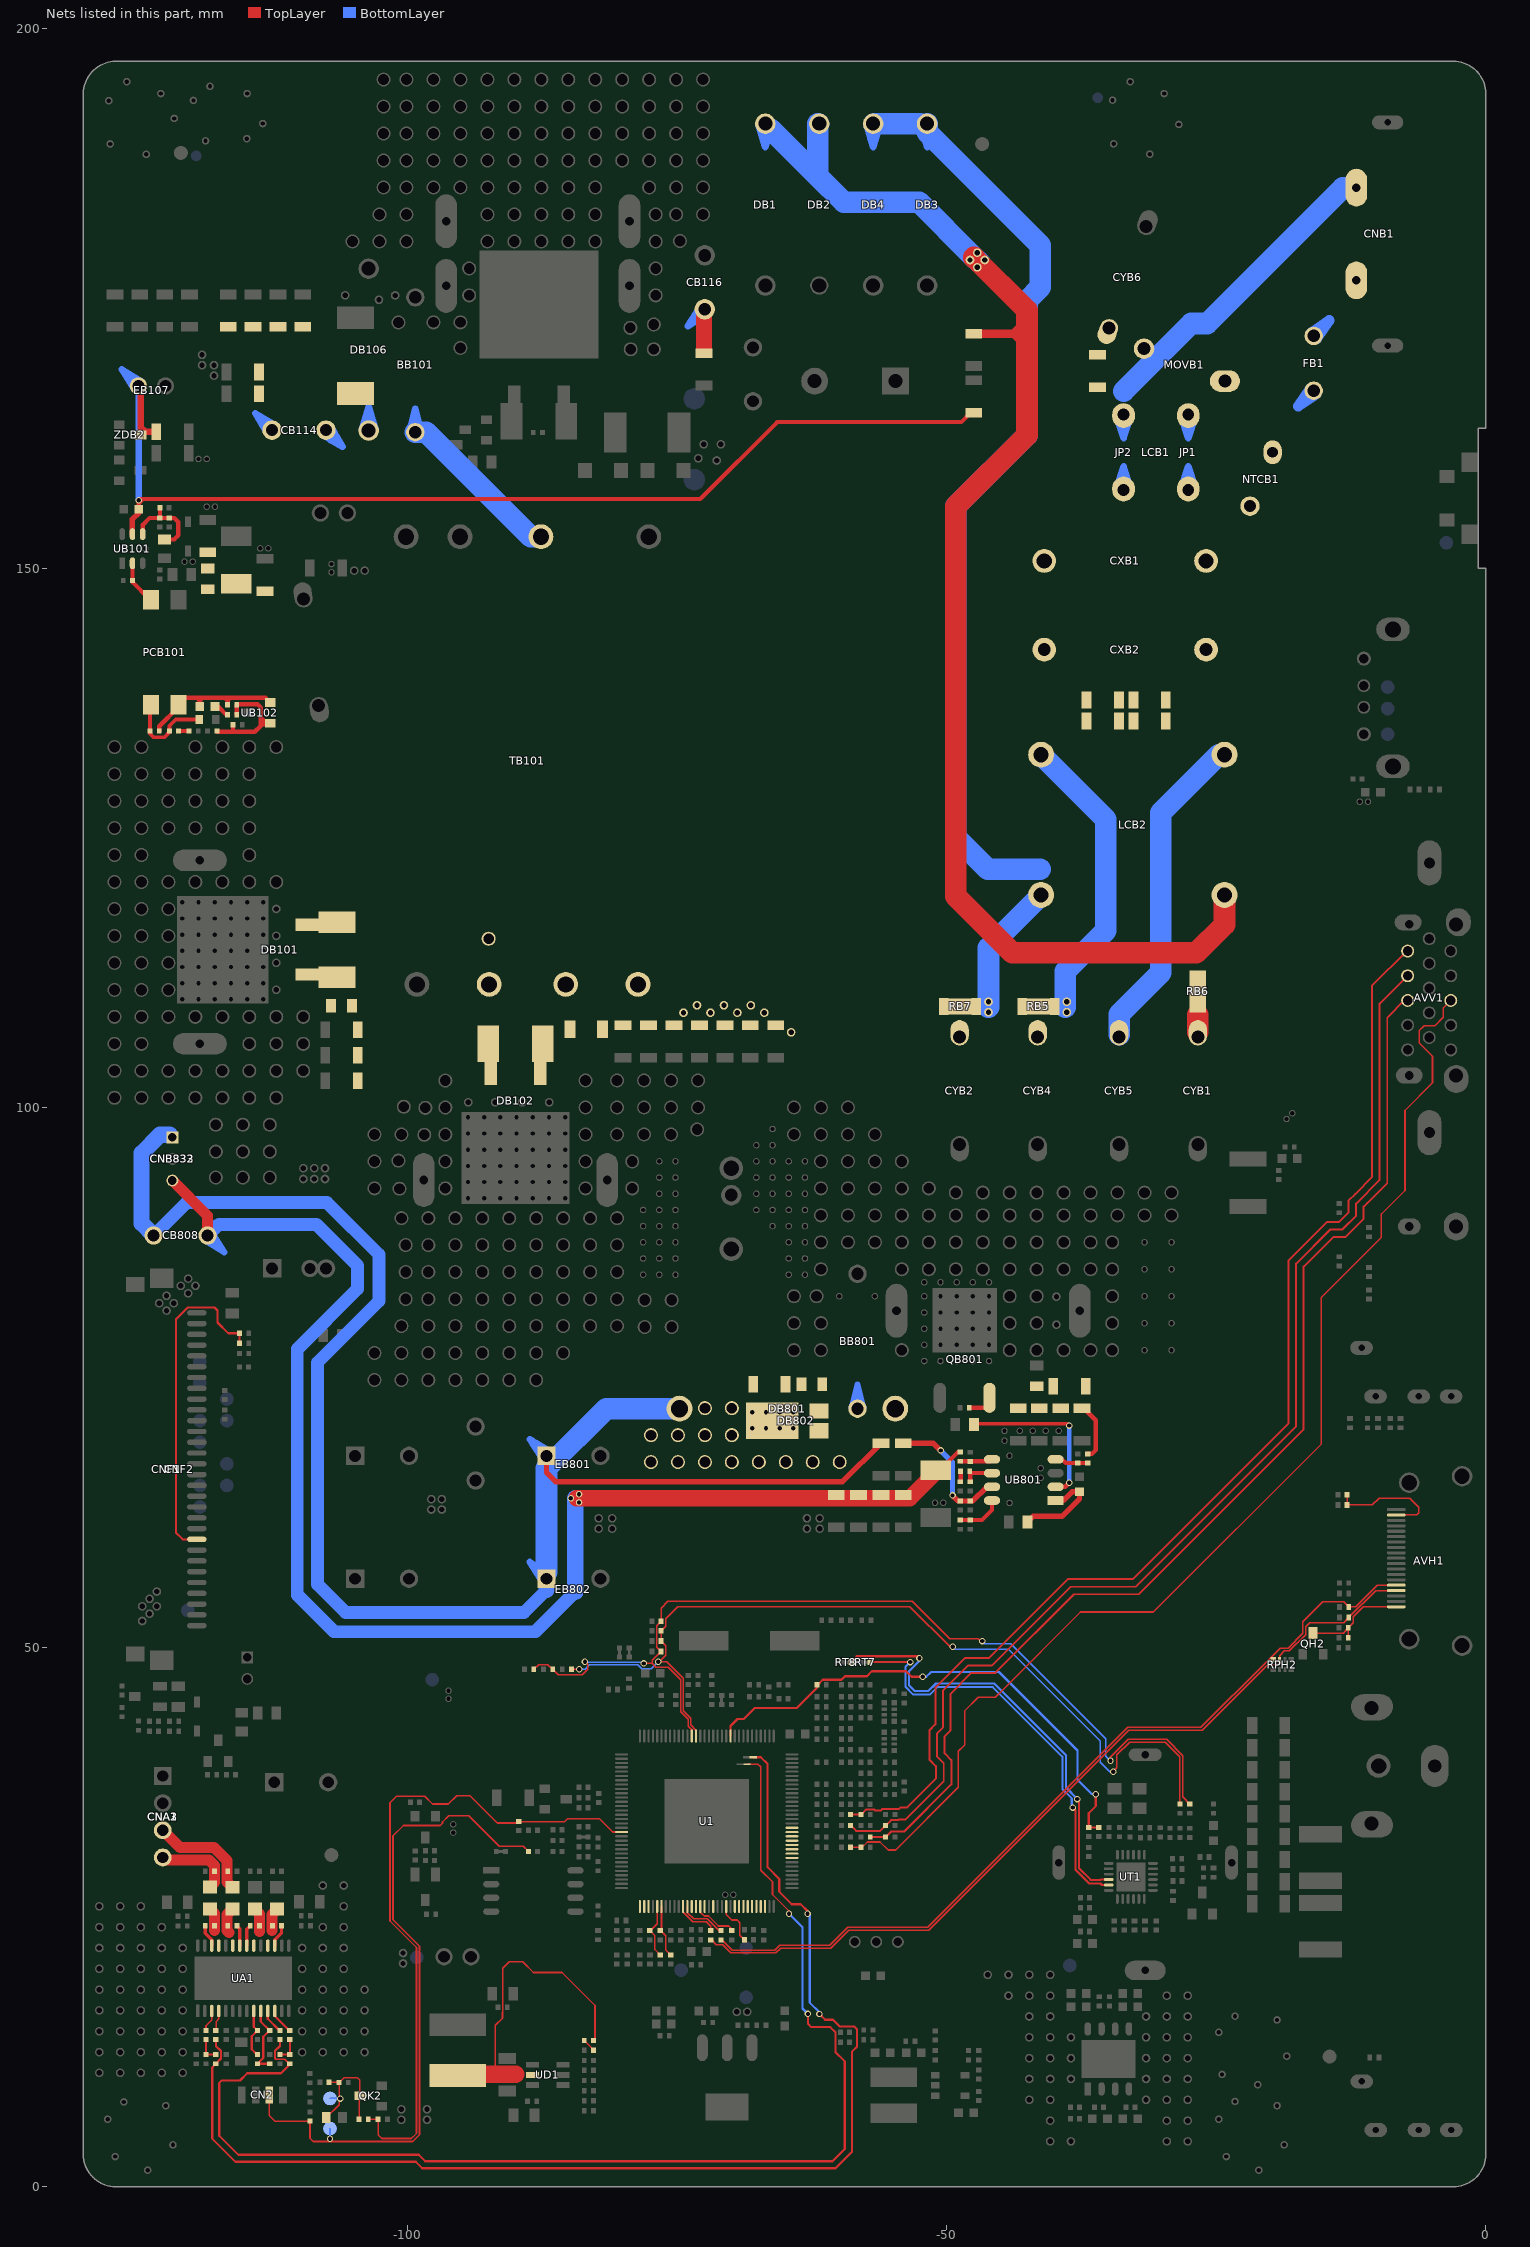
[diagram p0: the nets of this part, all layers, seen from the top]
# Altium PCB MISC84438.PcbDoc (part 11 of 15)
Units mm, origin at the board's own origin, x right, y up, seen from the top; angles counter-clockwise.
Board outline 130 x 197 mm, 2 copper layers (TopLayer, BottomLayer), stack 1.571 mm thick; 574 components, 314 nets, 2636 pads, 811 vias.

## Via types
v1: diameter 0.6, hole 0.4, TopLayer to BottomLayer, tented both sides, 780 vias
v2: diameter 0.7, hole 0.5, TopLayer to BottomLayer, tented both sides, 15 vias
v3: diameter 0.8, hole 0.6, TopLayer to BottomLayer, tented both sides, 12 vias
v4: diameter 0.8, hole 0.5, TopLayer to BottomLayer, tented both sides, 4 vias

## Nets (pads, with @x,y where several pads share a name; then routed paths per layer and width w, separated by ;. In a path a pad name is that pad's centre, name@x,y a point inside that pad or via, vN(x,y) a via of type N, cw(c..) or ccw(c..) an arc to the next point about the centre after c; other vN are vias at no path point) (continued)
HDMI1_SCL: RH10.1 U1.108 | length 4.4
  TopLayer w0.127: U1.108@-74.012,25.971 -74.012,25.406 -73.427,24.821 -72.17,24.821 -71.075,23.727 RH10.1@-70.891,23.727
HDMI1_SCL/: AVH1.15 DH6.K RH10.2 RPH2.2 | length 78
  TopLayer w0.127: RH10.2@-70.828,22.877 -69.875,21.924 -65.908,21.924 -65.47,22.362 -60.804,22.362 -59.137,24.028 -51.75,24.028 -49.472,26.307 -33.208,42.57 -26.409,42.57 -20.405,48.574 -19.064,49.915 -18.333,49.915 -16.968,51.28 -16.968,52.37 -15.787,53.552 -15.126,54.212 -13.172,54.212 DH6.K@-12.707,53.746 -12.075,53.746 -10.072,55.75 AVH1.15@-8.3,55.75
HDMI1_SDA: RH11.1 U1.107 | length 4
  TopLayer w0.127: U1.107@-74.412,25.971 -74.412,25.447 -73.532,24.567 -72.275,24.567 -71.831,24.123 RH11.1@-71.831,23.727
HDMI1_SDA/: AVH1.16 DH7.K RH11.2 RPH2.4 | length 78.7
  TopLayer w0.127: RH11.2@-71.755,22.877 -71.316,22.438 -70.749,22.438 -69.98,21.67 -65.803,21.67 -65.365,22.108 -60.699,22.108 -59.032,23.774 -58.162,23.774 -51.645,23.774 -33.103,42.316 -26.304,42.316 -20.223,48.396 -19.269,48.396 -19.122,48.543 RPH2.4@-19.122,48.837 -19.122,49.229 -18.69,49.661 -18.228,49.661 -16.714,51.175 -16.714,51.906 -16.33,52.29 -13.172,52.29 DH7.K@-12.707,52.756 -10.213,55.25 AVH1.16@-8.3,55.25
HDMI2_CLKN: U1.8
HDMI2_CLKP: U1.9@-64.312,30.871
HDMI2_HPDIN: U1.114
HDMI2_RX0N: U1.10
HDMI2_RX0P: U1.11
HDMI2_RX1N: U1.12
HDMI2_RX1P: U1.13
HDMI2_RX2N: U1.14
HDMI2_RX2P: U1.15
HDMI2_SCL: U1.110
HDMI2_SDA: U1.109
HDMI3_CLKN: U1.119
HDMI3_CLKP: U1.120
HDMI3_HPDIN: U1.112
HDMI3_RX0N: U1.121
HDMI3_RX0P: U1.122
HDMI3_RX1N: U1.123
HDMI3_RX1P: U1.124
HDMI3_RX2N: U1.125
HDMI3_RX2P: U1.126
HDMI3_SCL: U1.99
HDMI3_SDA: U1.98
HDMI_ARC: CH15.2 U1.117 | length 4.2
  TopLayer w0.152: U1.117@-70.412,25.971 -70.412,25.228 -69.896,24.711 -69.4,24.711 -69.154,24.465 -69.154,23.3 CH15.2@-68.726,22.872 CH15.2@-68.638,22.872
HDMI_CEC: RH13.2 U1.111 | length 4.1
  TopLayer w0.152: U1.111@-72.812,25.971 -72.812,25.441 -72.459,25.088 -72.059,25.088 -71.129,24.157 -70.179,24.157 RH13.2@-69.913,23.892
HDMI_DET: RH28.1 RH29.1 U1.102 | length 5
  TopLayer w0.152: RH29.1@-76.517,23.727 -76.412,23.832 U1.102@-76.412,25.971 ; RH29.1@-76.438,23.756 -76.467,23.727 -76.006,23.266 -76.006,21.932 RH28.1@-75.553,21.479
HDMI_PIN2: AVH1.2 DH2.K RH1.1 | length 10.9
  TopLayer w0.152: RH1.1@-12.859,64.135 DH2.K@-12.859,63.195 -10.516,63.195 -9.891,63.82 -7.05,63.82 -6.21,62.981 -6.21,62.454 -6.401,62.264 AVH1.2@-8.286,62.264
HOTPLUG1: AVH1.19 CH8.2 QH2.C RH14.1 | length 10
  TopLayer w0.127: QH2.C@-16.015,51.36 -15.955,51.3 -14.097,51.3 -14.08,51.317 -13.231,51.317 CH8.2@-12.758,51.791 ; RH14.1@-12.758,50.876 CH8.2@-12.758,51.791 ; AVH1.19@-8.3,53.75 -11.353,53.75 -12.27,52.833 -12.27,52.278 CH8.2@-12.758,51.791
HS_VGA: AVV1.13 RV12.1 RV13.1 | length 111.2
  TopLayer w0.152: RV12.1@-58.884,31.47 RV13.1@-57.905,31.47 ; RV13.1@-57.905,31.445 -57.818,31.445 -57.314,31.948 -56.154,31.948 -55.404,31.198 -54.709,31.198 -48.895,37.012 -48.895,40.35 -48.317,40.928 -48.317,44.082 -47.048,45.352 -45.477,45.352 ; -45.477,45.359 -45.47,45.359 -44.808,46.022 -37.565,53.264 -30.819,53.264 -15.24,68.842 -15.24,82.441 -9.677,88.004 -9.677,88.494 -9.677,90.156 -7.493,92.34 -7.493,99.758 -4.941,102.309 -4.941,104.778 -6.165,106.001 -6.165,107.17 -5.715,107.62 -4.71,107.62 -3.937,108.393 -3.937,109.26 AVV1.13@-3.247,109.95
IFAGC: CT19.2 RT2.2 RT18.2 U1.43 | length 48.1
  TopLayer w0.203: U1.43@-70.012,41.771 -70.012,42.698 -69.359,43.352 -68.799,43.352 -67.796,44.354 -63.89,44.354 -61.995,46.25 CT19.2@-61.995,46.507 -61.943,46.507 -61.46,46.99 -59.719,46.99 -59.392,47.316 -57.367,47.316 -56.912,47.771 -53.74,47.771 -53.226,47.257 v1(-52.197,47.257) ; v1(-36.153,36.381) -36.153,35.272 -36.804,34.621 RT2.2@-36.804,33.305 -36.792,33.293 RT18.2@-35.89,33.293 RT18.2@-35.954,33.357
  BottomLayer w0.203: v1(-52.197,47.257) -51.859,47.257 -51.415,47.701 -50.571,47.701 -45.121,47.701 -37.855,40.435 -37.855,37.73 -36.507,36.381 v1(-36.153,36.381)
IFn: RT8.1 UT1.16 | length 41.6
  TopLayer w0.203: RT8.1@-58.87,48.59 -58.303,49.157 -52.687,49.157 v1(-52.502,48.971) ; v1(-37.859,35.928) -37.706,35.776 -37.706,29.515 -36.627,28.435 -35.712,28.435 -35.684,28.464 UT1.16@-34.956,28.464
  BottomLayer w0.203: -52.807,48.438 -52.806,48.437 -53.462,47.781 -53.462,46.464 -52.934,45.936 -51.671,45.936 -50.973,46.634 -45.563,46.634 -38.922,39.993 -38.922,36.991 v1(-37.859,35.928) ; -52.807,48.439 -52.502,48.744 v1(-52.502,48.971)
IFp: RT7.1 UT1.17 | length 38.6
  TopLayer w0.203: RT7.1@-57.067,48.59 -57.029,48.628 v1(-53.365,48.628) ; v1(-38.303,35.141) -38.036,34.874 -38.036,29.378 -36.764,28.105 -35.712,28.105 -35.571,27.964 UT1.17@-34.956,27.964
  BottomLayer w0.203: v1(-53.365,48.628) -53.792,48.201 -53.792,46.328 -53.07,45.606 -51.534,45.606 -50.836,46.304 -45.7,46.304 -39.252,39.856 -39.252,37.262 -39.252,36.855 -38.387,35.99 -38.387,35.225 v1(-38.303,35.141)
IR: CN2.3 IR.1 RK15.2 RK16.2 | length 62.5
  TopLayer w0.152: CN2.3@-112.765,8.502 -112.765,6.593 -112.249,6.077 RK15.2@-108.991,6.077 -108.991,4.483 -108.687,4.178 -99.479,4.178 -98.841,4.817 -98.841,22.277 -101.295,24.732 -101.295,32.512 -100.33,33.477 -96.915,33.477 -96.71,33.682 -96.71,33.803 -96.13,34.384 -94.289,34.384 -91.452,31.547 -89.224,31.547 RK16.2@-88.741,31.064
  BottomLayer w0.152: v1(-107.137,4.445) IR.1@-107.137,5.385
KEY1: CK2.1 RK3.1 U1.101 | length 5.3
  TopLayer w0.152: CK2.1@-77.635,23.727 CK2.1@-77.559,23.803 ; U1.101@-76.812,25.971 -76.812,24.366 -77.451,23.727 CK2.1@-77.483,23.727 -77.021,23.265 -77.021,21.982 RK3.1@-76.517,21.479
L: DB1.K DB2.A LCB2.4 pad.VIA5@-46.449,178.588 pad.VIA5@-47.132,177.906 pad.VIA5@-47.132,179.271 pad.VIA5@-47.814,178.588 RB6.1 RB101.1 | length 132.8
  TopLayer w0.762: RB101.1@-47.6,171.756 RB101.1@-47.473,171.756 -43.764,171.756 ; -42.585,171.756 -43.764,171.756 ; -42.532,170.524 -43.764,171.756 ; -42.532,172.988 -43.764,171.756
  TopLayer w2: -47.441,178.822 -42.532,173.914 -42.532,172.988 -42.532,170.524 -42.532,162.344 -49.133,155.744 -49.133,119.593 -43.911,114.371 -26.829,114.371 -24.222,116.978 LCB2.4@-24.222,119.731
  BottomLayer w2: DB1.K@-66.273,190.707 -61.925,186.36 ; DB2.A@-61.906,191.222 -61.925,191.203 -61.925,189.472 -61.925,186.36 ; -46.863,178.273 -47.496,178.906 -52.515,183.925 -59.49,183.925 -61.925,186.36
L-1: CNB1.1@-12,176.7 FB1.1
L-2: FB1.2 NTCB1.2@-19.762,160.768
L-3: JP1.2 LCB1.1 MOVB1.1 NTCB1.1
L-4: CXB1.1 CXB2.2 CYB5.1 JP1.1@-27.582,157.263 LCB1.4 LCB2.1 RB1.1 RB2.1 | length 29.8
  BottomLayer w2: CYB5.1@-33.985,106.782 -33.985,108.687 -30.144,112.528 -30.144,127.34 LCB2.1@-24.753,132.731
L-5: CYB1.1 RB6.2 RB6.3 | length 1.6
  TopLayer w2: CYB1.1@-26.691,106.991 -26.691,108.609
L-N: RB1.2 RB2.2 RB3.1 RB4.1
LED+: CB808.2 CNB832.1 CNB833.1 DB801.K DB802.2 EB801.1@-87.073,67.742 EB802.1@-87.073,56.35 pad.VIA5@-59.89,67.158 pad.VIA5@-62.39,67.158 pad.VIA5@-64.89,67.158 pad.VIA5@-64.187,70.284 pad.VIA5@-64.187,71.784 pad.VIA5@-65.459,70.284 pad.VIA5@-65.459,71.784 pad.VIA5@-66.73,70.284 pad.VIA5@-66.73,71.784 pad.VIA5@-67.39,67.158 pad.VIA5@-68.001,70.284 pad.VIA5@-68.001,71.784 pad.VIA5@-69.89,67.158 pad.VIA5@-69.89,69.658 pad.VIA5@-69.89,72.158 pad.VIA5@-72.39,67.158 pad.VIA5@-72.39,69.658 pad.VIA5@-72.39,72.158 pad.VIA5@-74.89,67.158 pad.VIA5@-74.89,69.658 pad.VIA5@-77.39,67.158 pad.VIA5@-77.39,69.658 RB812.2 RB814.1 | length 150.7
  TopLayer w0.5: EB801.1@-87.073,67.742 -87.073,66.195 -86.22,65.341 -59.639,65.341 -56.082,68.899 RB814.1@-56.069,68.899
  BottomLayer w1.2: CB808.2@-123.483,88.168 -120.438,91.214 -107.414,91.214 -102.6,86.4 -102.6,82.1 -108.306,76.394 -108.306,55.829 -105.689,53.213 -89.164,53.213 -87.073,55.303
  BottomLayer w1.5: CB808.2@-123.483,88.168 -124.6,89.285 -124.6,95.8 -122.9,97.5 CNB832.1@-122,97.5 ; -87.073,55.303 EB802.1@-87.073,56.35
  BottomLayer w2: EB802.1@-87.073,56.933 -87.073,66.572 -81.531,72.114 DB801.K@-75.342,72.114
LED_CS: QB801.S RB806.2 RB808.1 RB810.2 RB818.1 RB819.1 RB820.1 RB821.1 | length 6.6
  TopLayer w0.4: RB808.1@-47.886,72.2 -46.685,72.2 ; RB818.1@-37.423,72.15 -37.276,72.15 -36.157,71.031 -36.157,68.275 -36.511,67.921 RB806.2@-36.893,67.921
LED_FB: CB808.1 CNB832.3 CNB833.3 DB804.A pad.VIA5@-84.049,63.424 pad.VIA5@-84.049,64.186 pad.VIA5@-84.811,63.805 RB805.2 RB837.2 RB838.2 RB839.1 RB840.2 | length 129.1
  TopLayer w0.4: DB804.A@-50.592,66.424 -48.925,68.091 RB805.2@-48.73,68.091
  TopLayer w1: CNB832.3@-121.744,93.263 -118.483,90.002 CB808.1@-118.483,88.468
  TopLayer w1.5: -84.277,63.805 -53.391,63.805 DB804.A@-50.99,66.205
  BottomLayer w1.2: CB808.1@-118.483,88.168 -117.447,89.205 -108.405,89.205 -104.6,85.4 -104.6,83.2 -110.176,77.624 -110.176,54.855 -106.756,51.435 -88.101,51.435 -84.405,55.131
  BottomLayer w1.5: -84.405,55.131 -84.405,63.805
LED_GATE: RB807.1 UB801.2 | length 15.7
  TopLayer w0.3: RB807.1@-47.445,70.65 -47.388,70.706 -38.779,70.706 v1(-38.621,70.549)
  TopLayer w0.4: UB801.2@-39.874,64.872 -38.989,64.872 v1(-38.621,65.24)
  BottomLayer w0.4: v1(-38.621,65.24) v1(-38.621,70.549) v1@-38.621,70.65
LED_OVP: CB806.1 RB803.2 RB835.2 UB801.7 | length 12.3
  TopLayer w0.5: RB835.2@-53.993,68.899 -51.195,68.899 v1(-50.533,68.237) ; v1@-50.54,68.231 v1@-50.533,68.224 ; v1(-49.433,64.072) -48.918,63.557 RB803.2@-48.73,63.557 -47.568,63.557 UB801.7@-46.253,64.872
  BottomLayer w0.5: v1(-50.533,68.237) -49.433,67.137 v1(-49.433,64.072)
LED_R: CK10.2 DK20.A LED.1 QK2.C RK1.1 RK21.2 | length 11.5
  TopLayer w0.152: DK20.A@-107.479,6.417 -106.292,7.604 CK10.2@-106.292,9.652 ; RK1.1@-107.22,9.677 -106.318,9.677 CK10.2@-106.292,9.652 ; RK21.2@-104.438,6.248 -104.438,8.402 QK2.C@-104.42,8.42 ; QK2.C@-104.356,8.42 QK2.C@-104.42,8.42 ; CK10.2@-106.292,9.652 -105.839,10.105 -104.593,10.105 -104.381,9.893 -104.381,8.459 QK2.C@-104.42,8.42
  BottomLayer w0.152: LED.1@-107.137,8.179 -106.21,8.179 v1(-106.197,8.166)
LED_RED: RK18.1 RK20.2 RK21.1 U1.83 | length 62
  TopLayer w0.152: RK21.1@-103.588,6.248 RK20.2@-102.673,6.248 -102.673,4.794 -102.337,4.458 -99.595,4.458 -99.12,4.933 -99.12,22.162 -101.575,24.616 -101.575,35.597 -100.976,36.195 -98.362,36.195 -97.63,35.463 -96.169,35.463 -95.399,36.233 -94.163,36.233 -91.636,33.706 -89.782,33.706 RK18.1@-89.664,33.824 ; RK18.1@-89.637,33.851 RK18.1@-89.664,33.824 ; U1.83@-80.112,32.871 -80.919,32.871 -82.162,34.113 -85.115,34.113 -85.405,33.824 RK18.1@-89.664,33.824
LOUT+: CA4.1 CNA1.4 CNA2.4 CNA3.4 LBA1.2 | length 7.3
  TopLayer w1.016: CNA2.4@-122.636,30.51 -122.403,30.277 -118.355,30.277 -117.839,29.761 -117.839,28.21 LBA1.2@-118.274,27.775
LOUT-: CA5.1 CNA1.3 CNA2.3 CNA3.3 LBA2.2 | length 9.8
  TopLayer w1.016: CNA2.3@-122.636,33.03 -121.026,31.42 -117.881,31.42 -116.696,30.235 -116.696,28.254 LBA2.2@-116.191,27.749
LVDS_SEL: CNF1.22 CNF2.22 RF20.1 RF21.2 | length 30.9
  TopLayer w0.203: CNF2.22@-119.486,60 -120.797,60 -121.415,60.617 -121.415,80.398 -120.313,81.499 -117.851,81.499 -117.557,81.205 -117.557,80.107 -116.559,79.109 RF21.2@-115.518,79.109 ; RF20.1@-115.518,78.169 RF21.2@-115.518,79.109 ; RF21.2@-115.518,79.165 RF21.2@-115.518,79.109
M_SCL: DT3.K RF23.1 RF25.1 RT3.2 RT6.1 U1.52 | length 89.8
  TopLayer w0.127: RF23.1@-88.246,47.955 -87.806,48.396 -86.953,48.396 -86.512,47.955 RF25.1@-86.494,47.955 -85.998,47.46 -83.775,47.46 -83.261,47.974 -83.261,48.41 v1(-83.502,48.651) ; v1(-78.041,48.499) -77.267,48.499 ; DT3.K@-76.454,49.496 DT3.K@-76.454,49.603 ; U1.52@-73.612,41.771 -73.612,42.364 -73.939,42.691 -73.939,43.311 -74.642,44.013 -74.642,47.007 -75.8,48.164 -76.933,48.164 -77.267,48.499 ; v1(-46.672,50.571) -46.824,50.571 -47.035,50.782 -49.694,50.782 -53.178,54.267 -75.814,54.267 -76.454,53.627 RT3.2@-76.454,52.417 -76.87,52.001 -76.87,50.019 DT3.K@-76.454,49.603 ; v1(-34.791,39.467) -34.791,39.802 -33.134,41.459 -29.597,41.459 -28.099,39.96 -28.099,36.118 RT6.1@-27.445,35.464 ; -77.267,48.499 -77.267,48.816 -76.479,49.603 DT3.K@-76.454,49.603
  BottomLayer w0.127: v1@-83.502,48.616 -78.159,48.616 v1(-78.041,48.499) ; v1(-46.672,50.571) -46.431,50.33 -44.033,50.33 -35.226,41.524 -35.226,39.902 v1(-34.791,39.467)
M_SDA: DT2.K RF27.1 RT4.2 RT5.1 U1.51 | length 84.4
  TopLayer w0.127: RF27.1@-84.767,47.955 cw(c-84.733,47.921) -84.733,47.969 v1(-84.036,47.969) ; v1(-76.721,48.664) v1@-76.624,48.664 ; U1.51@-73.212,41.771 -73.212,42.323 -73.685,42.796 -73.685,43.416 -73.774,43.505 -74.388,44.119 -74.388,47.112 -75.94,48.664 v1@-76.624,48.664 ; v1(-49.416,50.038) -49.668,50.038 -53.389,53.759 -74.919,53.759 -76.038,52.64 -76.038,51.93 RT4.2@-76.454,51.515 DT2.K@-76.454,50.569 -76.038,50.153 -76.038,49.249 v1@-76.624,48.664 ; v1(-34.544,38.468) -34.196,38.816 -34.196,40.038 -33.029,41.205 -29.703,41.205 -28.353,39.855 RT5.1@-28.353,35.47
  BottomLayer w0.127: v1(-84.036,47.969) -83.49,47.969 -83.098,48.362 -78.598,48.362 -78.245,48.008 -77.376,48.008 v1(-76.721,48.664)
  BottomLayer w0.152: v1(-49.416,50.038) -49.187,49.809 -44.248,49.809 -35.747,41.308 -35.747,39.352 -34.863,38.468 v1(-34.544,38.468)
MHL_CABLE_DET: U1.97
N: DB3.K DB4.A LCB2.3 pad.VIA5@-46.101,108.865 pad.VIA5@-46.101,109.83 RB7.1 | length 100.4
  BottomLayer w2: DB4.A@-56.67,191.222 -52.422,191.222 DB3.K@-51.788,190.588 ; DB3.K@-51.788,191.222 -51.788,191.09 -51.788,191.027 -51.788,190.874 -51.788,190.773 DB3.K@-51.788,190.588 ; -46.101,109.347 -46.101,114.853 LCB2.3@-41.222,119.731 ; -41.3,122.1 -46.167,122.1 -49.133,125.066 -49.133,155.744 -42.532,162.344 -42.532,174.828 -41.288,176.073 -41.288,179.946 -51.455,190.113 -51.788,190.447 DB3.K@-51.788,190.588
N-1: CNB1.2 JP2.2 LCB1.2 MOVB1.2@-31.682,170.366 RB8.1 | length 29.2
  BottomLayer w2: -33.582,166.418 -27.3,172.7 -25.84,172.7 -13.24,185.3 ; -13.04,185.3 CNB1.2@-12,185.3
N-2: CXB1.2 CXB2.1 JP2.1@-33.582,157.263 LCB1.3 LCB2.2 pad.VIA5@-38.837,108.865 pad.VIA5@-38.837,109.83 RB3.2 RB4.2 RB5.1 | length 27.4
  BottomLayer w2: LCB2.2@-41.222,132.731 -35.244,126.753 -35.244,116.394 -38.985,112.653 -38.985,109.322
N-4: CYB2.1 RB7.2 RB7.3
N-5: CYB4.1 RB5.2 RB5.3
N-6: CYB6.1 RB8.2
NetAVV1_1: AVV1.1 RV1.2 RV2.2 | length 110.2
  TopLayer w0.18: RV1.2@-58.884,34.493 RV2.2@-57.905,34.493 -57.438,34.96 -56.698,34.96 -56.602,34.865 -56.085,34.865 -55.959,34.991 -54.405,34.991 -54.24,35.155 -53.652,35.155 -50.977,37.831 -50.977,38.981 -51.568,39.573 -51.568,42.308 -51.029,42.847 -51.029,46.241 -48.26,49.009 -46.049,49.009 -38.753,56.305 -32.742,56.305 -18.282,70.766 -18.282,85.853 -14.715,89.419 -13.598,89.419 -12.719,90.298 -12.719,91.415 -12.126,92.009 -10.535,93.6 -10.535,111.346 -7.351,114.53 AVV1.1@-7.247,114.53
NetAVV1_2: AVV1.2 RV3.2 RV5.2 | length 109.2
  TopLayer w0.18: RV3.2@-58.884,33.477 -58.377,32.969 -56.139,32.969 RV5.2@-55.632,33.476 -55.134,33.974 -54.476,33.974 -54.4,34.049 -53.77,34.049 -50.248,37.572 -50.248,39.24 -50.87,39.862 -50.87,42.018 -50.33,42.558 -50.33,45.951 -47.971,48.311 -45.76,48.311 -38.464,55.607 -32.452,55.607 -17.583,70.476 -17.583,85.564 -14.426,88.721 -13.309,88.721 -12.021,90.009 -12.021,91.126 -9.836,93.311 -9.836,109.651 AVV1.2@-7.247,112.24
NetAVV1_3: AVV1.3 RV9.2 RV11.2 | length 105.9
  TopLayer w0.18: RV9.2@-57.055,32.41 RV11.2@-55.632,32.41 -55.124,32.918 -53.913,32.918 -49.549,37.282 -49.549,39.529 -50.171,40.152 -50.171,41.729 -49.632,42.269 -49.632,45.662 -47.681,47.612 -45.471,47.612 -38.175,54.908 -32.163,54.908 -16.885,70.187 -16.885,85.274 -14.137,88.022 -13.019,88.022 -11.322,89.719 -11.322,90.837 -10.998,91.161 -9.138,93.021 -9.138,108.361 -7.549,109.95 AVV1.3@-7.247,109.95
NetBB101_2: BB101.2 TB101.3 | length 15.7
  BottomLayer w2: BB101.2@-99.228,162.624 -98.209,162.624 -88.528,152.943 TB101.3@-87.585,152.943
NetBB801_2: BB801.2 CB810.1 DB801.A DB802.1 DB802.3
NetCA6_1: CA6.1 UA1.3 | length 2
  TopLayer w0.152: CA6.1@-118.629,14.482 -118.629,14.924 -118.1,15.453 UA1.3@-118.1,16.29
NetCA6_2: CA6.2 CA27.1 RA21.2 | length 2.3
  TopLayer w0.203: CA6.2@-118.629,13.632 RA21.2@-118.629,12.247 CA27.1@-117.715,12.247
NetCA7_1: CA7.1 UA1.26 | length 2.2
  TopLayer w0.305: CA7.1@-118.626,24.106 CA7.1@-118.699,24.179 -118.699,23.496 -118.1,22.897 UA1.26@-118.1,22.34
NetCA7_2: CA7.2 LBA1.1 UA1.25 | length 2.2
  TopLayer w1.016: LBA1.1@-118.274,25.743 -117.839,25.308 -117.839,23.754
NetCA8_1: CA8.1 UA1.4 | length 1.9
  TopLayer w0.152: CA8.1@-117.715,14.482 -117.691,14.506 -117.691,15.316 -117.45,15.557 UA1.4@-117.45,16.29
NetCA8_2: CA8.2 CA27.2 RA2.JP_1K | length 113.4
  TopLayer w0.203: CA8.2@-117.715,13.632 -117.715,13.045 -117.236,12.566 -117.236,11.875 CA27.2@-117.715,11.397 -118.059,11.052 -118.059,4.451 -115.907,2.299 -99.18,2.299 -98.583,1.702 -60.28,1.702 -58.763,3.219 -58.763,12.509 -58.293,12.979 -58.293,14.585 -58.548,14.84 -59.884,14.84 -60.518,15.473 -61.244,15.473 v1(-61.773,16.002) ; RA2.JP_1K@-67.903,39.802 -67.198,39.802 -66.573,39.177 -66.573,29.597 -65.492,28.516 -65.492,27.346 -64.331,26.185 -63.514,26.185 v1@-62.874,25.544
  BottomLayer w0.203: v1(-62.874,25.291) -62.833,25.291 -62.676,25.133 -62.676,17.058 -61.773,16.155 v1(-61.773,16.002)
NetCA12_1: CA12.1 UA1.22 | length 1.9
  TopLayer w0.305: CA12.1@-115.766,24.178 -115.5,23.912 UA1.22@-115.5,22.34
NetCA12_2: CA12.2 LBA2.1 UA1.23 | length 2.5
  TopLayer w1.016: -116.51,23.55 -116.696,23.735 -116.696,25.213 LBA2.1@-116.191,25.717
NetCA13_1: CA13.1 UA1.21 | length 2
  TopLayer w0.305: UA1.21@-114.85,22.34 -114.85,23.862 CA13.1@-114.533,24.179
NetCA13_2: CA13.2 LBA3.1 UA1.20 | length 2.2
  TopLayer w1.016: LBA3.1@-114.108,25.717 -113.673,25.282 -113.673,23.666
NetCA15_1: CA15.1 RA11.2 UA1.9 | length 4.6
  TopLayer w0.203: UA1.9@-114.2,16.29 -114.2,14.828 CA15.1@-113.854,14.482 -114.384,13.952 -114.384,12.735 -113.896,12.247 RA11.2@-113.854,12.247
NetCA18_1: CA18.1 RA11.1 RA12.1 UA1.10 | length 6.8
  TopLayer w0.203: UA1.10@-113.55,16.29 -113.55,15.295 CA18.1@-112.737,14.482 -113.327,13.892 -113.327,11.924 RA11.1@-113.854,11.397 RA12.1@-112.737,11.397
NetCA20_1: CA20.1 UA1.12 | length 2.4
  TopLayer w0.203: UA1.12@-112.25,16.29 -112.25,15.824 CA20.1@-110.908,14.482
NetCA20_2: CA20.2 CA29.1 RA5.2 | length 2.3
  TopLayer w0.203: RA5.2@-111.772,12.247 CA29.1@-110.857,12.247 CA20.2@-110.857,13.632
NetCA21_1: CA21.1 UA1.11 | length 2.3
  TopLayer w0.203: UA1.11@-112.9,16.29 -112.9,15.56 CA21.1@-111.822,14.482
NetCA21_2: CA21.2 CA29.2 RA15.JP_1K | length 116.2
  TopLayer w0.127: -112.145,11.822 -112.135,11.812 -111.331,11.812 -110.916,11.397 CA29.2@-110.857,11.397
  TopLayer w0.152: RA15.JP_1K@-68.489,39.167 -67.461,39.167 -67.208,38.914 -67.208,29.334 -66.127,28.253 -66.127,27.083 -64.592,25.547 v1(-64.592,25.296)
  TopLayer w0.203: -112.145,11.822 -112.25,11.927 -112.25,12.566 -111.771,13.045 CA21.2@-111.771,13.632 ; CA29.2@-110.857,11.397 -110.857,11.33 -111.684,10.503 -114.821,10.503 -115.485,9.838 -117.177,9.838 -117.399,9.617 -117.399,4.724 -115.634,2.959 -98.907,2.959 -98.31,2.362 -60.554,2.362 -59.423,3.492 -59.423,11.61 -60.283,12.47 -60.283,14.3 -60.771,14.788 -62.525,14.788 -62.835,15.097 v1(-62.836,16.004) v1(-62.836,16.004)
  BottomLayer w0.203: v1(-64.592,25.296) -63.336,24.039 -63.336,16.504 v1(-62.836,16.004)
NetCA22_1: CA22.1 UA1.17 | length 2.1
  TopLayer w0.305: UA1.17@-112.25,22.34 -112.25,22.89 -111.626,23.514 CA22.1@-111.626,24.178
NetCA22_2: CA22.2 LBA4.1 UA1.18 | length 2.2
  TopLayer w1.016: -112.53,23.724 -112.53,25.238 LBA4.1@-112.051,25.717
NetCB101_1: CB101.1 RB103.2 RB105.1 RB112.1 UB101.4 | length 8.1
  TopLayer w0.4: UB101.4@-124.5,153.177 -124.5,154.036 -123.857,154.679 CB101.1@-123.012,154.679 ; RB105.1@-122.904,155.613 -122.904,154.711 CB101.1@-122.936,154.679 RB103.2@-122.022,154.679 -121.583,154.679 -121.209,154.305 -121.209,153.06 -121.587,152.682 RB112.1@-122.479,152.682
NetCB102_1: CB102.1 EB107.1 RB102.2 RB111.1 UB101.5 ZDB2.2 | length 101.3
  TopLayer w0.4: CB102.1@-124.859,155.473 v1@-124.859,156.027 ; v1(-124.859,156.326) v1@-124.859,156.027 ; v1@-124.759,156.426 -124.46,156.426 ; RB102.2@-47.473,164.438 -47.753,164.438 -48.612,163.579 -65.668,163.579 -72.822,156.426 -124.46,156.426 ; v1@-124.859,156.027 -124.46,156.426
  TopLayer w0.5: UB101.5@-125.45,153.177 -125.45,154.56 -124.859,155.151 CB102.1@-124.859,155.473
  TopLayer w0.6: ZDB2.2@-124.688,162.369 -124.688,163.093 ; EB107.1@-124.688,166.702 -124.688,163.093 ; ZDB2.2@-124.403,162.655 ZDB2.2@-124.249,162.655 ; RB111.1@-123.242,162.655 ZDB2.2@-124.249,162.655 ; -124.688,163.093 ZDB2.2@-124.249,162.655
  BottomLayer w0.4: v1(-124.859,156.326) v1@-124.859,156.408
  BottomLayer w0.6: v1@-124.859,156.408 EB107.1@-124.859,166.916
NetCB103_1: CB103.1 PCB101.4 UB101.2 | length 4
  TopLayer w0.4: UB101.2@-125.45,150.477 -125.45,148.729 PCB101.4@-123.844,147.123
NetCB109_1: CB109.1 CB110.1 PCB101.2 RB132.1 UB102.K | length 15
  TopLayer w0.4: RB132.1@-122.968,134.929 -122.968,135.375 -121.18,137.163 PCB101.2@-121.18,137.347 -120.524,138.004 -116.371,138.004 -116.63,137.744 ; -119.47,137.991 -119.21,137.731 ; CB109.1@-119.21,137.198 -119.21,137.731 ; -119.21,137.935 -119.21,137.731 ; -118.951,137.991 -119.21,137.731 ; -116.89,138.004 -116.63,137.744 ; CB110.1@-116.63,137.351 -116.63,137.744 ; -116.63,137.966 -116.63,137.744 ; -116.271,138.004 -113.114,138.004 UB102.K@-112.575,137.465
NetCB109_2: CB109.2 RB133.2 | length 1
  TopLayer w0.4: CB109.2@-117.432,137.132 RB133.2@-116.723,136.423
NetCB110_2: CB110.2 RB133.1 RB134.2 RB135.2 UB102.R | length 12.6
  TopLayer w0.4: RB135.2@-117.56,134.856 -116.9,134.856 ; -116.49,134.856 -116.9,134.856 ; -116.271,134.856 -116.125,134.856 ; -116.125,134.931 RB134.2@-116.125,135.5 ; RB133.1@-115.78,136.423 CB110.2@-115.78,137.35 ; CB110.2@-115.631,137.4 -113.861,137.4 -113.546,137.085 -113.546,136.169 ; UB102.R@-112.575,135.56 UB102.R@-112.936,135.56 ; UB102.R@-112.549,135.534 UB102.R@-112.524,135.56 ; -116.9,134.856 -116.125,134.856 ; -116.125,134.856 -114.105,134.856 -113.546,135.415 ; -113.546,135.415 -113.546,135.89 ; -113.546,135.415 -113.401,135.56 -113.216,135.56 ; -113.546,135.89 -113.216,135.56 ; -113.546,135.89 -113.546,136.169 ; -113.546,136.169 UB102.R@-112.936,135.56 ; -113.216,135.56 UB102.R@-112.936,135.56
NetCB113_1: CB113.1 DB104.A RB114.1
NetCB113_2: CB113.2 RB116.1
NetCB114_1: CB114.1@-112.507,162.814 RB117.1 RB118.1
NetCB114_2: CB114.2 DB103.K DB106.K RB153.1 RB154.1 RB155.1 RB157.1
NetCB116_1: CB116.1 RB119.2 | length 3.7
  TopLayer w1.5: RB119.2@-72.477,170.258 CB116.1@-72.477,173.955
NetCB117_1: CB117.1 DB101.1 DB101.3 pad.VIA5@-92.431,115.672 TB101.7 TB101.9
NetCB117_2: CB117.2 RB128.1 RB129.1 RB165.1
NetCB118_1: CB118.1 DB102.1 DB102.3 TB101.8
NetCB118_2: CB118.2 pad.VIA5@-64.4,107 pad.VIA5@-66.871,108.814 pad.VIA5@-68.121,109.505 pad.VIA5@-69.371,108.814 pad.VIA5@-70.621,109.505 pad.VIA5@-71.871,108.814 pad.VIA5@-73.121,109.505 pad.VIA5@-74.371,108.814 RB124.1 RB125.1 RB126.1 RB127.1 RB162.1 RB163.1 RB164.1
NetCB125_1: CB125.1 PCB101.1 RB131.1 RB132.2 | length 8.4
  TopLayer w0.35: PCB101.1@-123.72,137.347 -123.818,137.249 RB132.2@-123.818,134.929 -123.818,134.689 -123.469,134.341 -122.504,134.341 -122.015,134.83 CB125.1@-122.015,134.925 -122.015,135.414 -121.437,135.992 RB131.1@-119.26,135.992
NetCB125_2: CB125.2 RB158.1 | length 1
  TopLayer w0.35: CB125.2@-121.165,134.925 RB158.1@-120.206,134.925
NetCB801_2: CB801.2 RB816.2 UB801.1 | length 9
  TopLayer w0.5: RB816.2@-42.489,61.595 -41.96,62.124 -39.297,62.124 -37.668,63.753 CB801.2@-37.668,64.407 -38.362,64.407 -39.167,63.602 UB801.1@-39.874,63.602 UB801.1@-40.006,63.602
NetCB803_1: CB803.1 RB806.1 UB801.4 | length 3.1
  TopLayer w0.4: UB801.4@-39.874,67.412 -39.281,67.412 -38.941,67.071 RB806.1@-36.893,67.071
NetCB804_1: CB804.1 RB805.1 UB801.5 | length 2.8
  TopLayer w0.4: RB805.1@-48.73,67.241 UB801.5@-45.945,67.241
NetCB805_2: CB805.2 RB804.1 | length 1
  TopLayer w0.4: CB805.2@-48.73,65.335 -48.685,65.38 RB804.1@-48.685,66.294
NetCB809_1: CB809.1 RB810.1
NetCB810_2: CB810.2 RB812.1
NetCB812_2: CB812.2 RB804.2 UB801.6 | length 2.8
  TopLayer w0.4: CB812.2@-47.803,65.335 -47.803,66.021 -47.683,66.142 UB801.6@-45.774,66.142
NetCB813_2: CB813.2 RB813.1 UB801.8 | length 4.2
  TopLayer w0.4: RB813.1@-48.73,61.791 -46.705,61.791 -45.774,62.722 UB801.8@-45.774,63.602
NetCD2_1: CD2.1 RD2.2 | length 1.3
  TopLayer w0.152: CD2.1@-83.571,13.551 -82.721,12.701 RD2.2@-82.721,12.625
NetCD2_2: CD2.2 LD3.1 UD1.2 | length 28.6
  TopLayer w0.127: -91.145,16.18 -91.145,16.939 -91.135,16.949
  TopLayer w0.152: -91.808,11.151 -91.808,14.948 -91.145,15.612 -91.145,16.18 ; -91.135,16.949 -91.135,20.231 -90.512,20.854 -89.28,20.854 -88.273,19.847 -85.632,19.847 -82.572,16.787 -82.572,13.7 CD2.2@-82.721,13.551
  TopLayer w1.651: LD3.1@-95.301,10.299 -95.176,10.424 -89.929,10.424